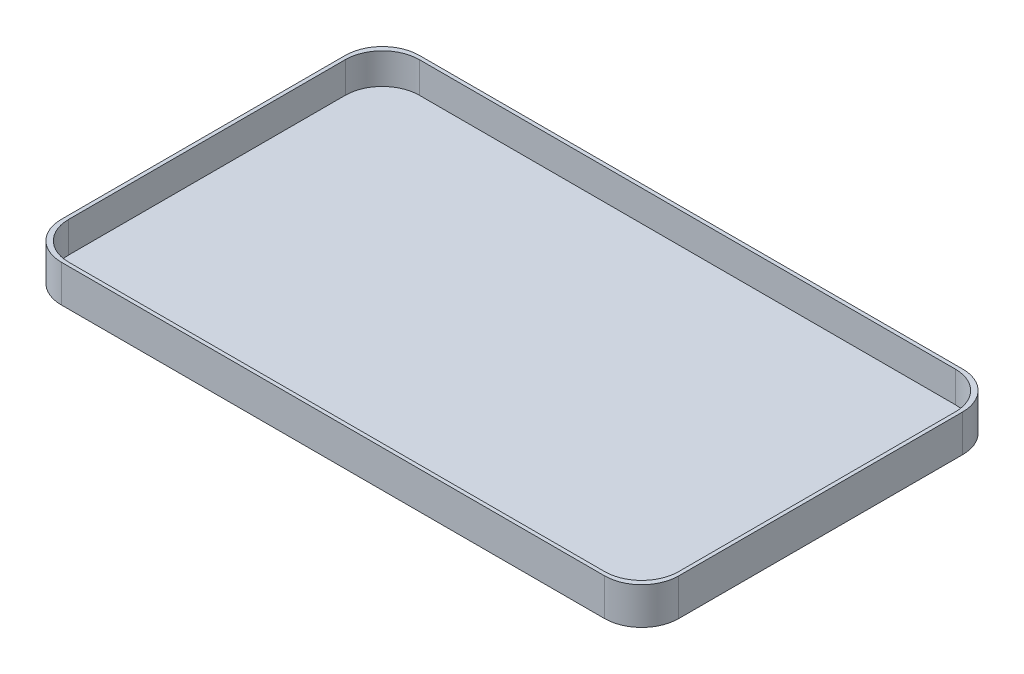
from build123d import *

# Parameters (mm, degrees)
BOSS_EXTRUDE1_DEPTH = 30
CUT_EXTRUDE1_DEPTH  = 25


with BuildPart() as part:
    # Sketch1 → Boss-Extrude1 (new body)
    with BuildSketch(Plane(origin=(0, 0, 0), x_dir=(1, 0, 0), z_dir=(0, 1, 0))):
        with BuildLine():
            Line((-220, 145), (220, 145))
            ThreePointArc((220, 145), (241.213203436, 136.213203436), (250, 115))
            Line((250, 115), (250, -115))
            ThreePointArc((250, -115), (241.213203436, -136.213203436), (220, -145))
            Line((220, -145), (-220, -145))
            ThreePointArc((-220, -145), (-241.213203436, -136.213203436), (-250, -115))
            Line((-250, -115), (-250, 115))
            ThreePointArc((-250, 115), (-241.213203436, 136.213203436), (-220, 145))
        make_face()
    extrude(amount=BOSS_EXTRUDE1_DEPTH)

    # Sketch2 → Cut-Extrude1 (cut)
    with BuildSketch(Plane(origin=(0, 30, 0), x_dir=(1, 0, 0), z_dir=(0, 1, 0))):
        with BuildLine():
            Line((-217, 142), (217, 142))
            ThreePointArc((217, 142), (238.213203436, 133.213203436), (247, 112))
            Line((247, 112), (247, -112))
            ThreePointArc((247, -112), (238.213203436, -133.213203436), (217, -142))
            Line((217, -142), (-217, -142))
            ThreePointArc((-217, -142), (-238.213203436, -133.213203436), (-247, -112))
            Line((-247, -112), (-247, 112))
            ThreePointArc((-247, 112), (-238.213203436, 133.213203436), (-217, 142))
        make_face()
    extrude(amount=-CUT_EXTRUDE1_DEPTH, mode=Mode.SUBTRACT)


solid = part.part
